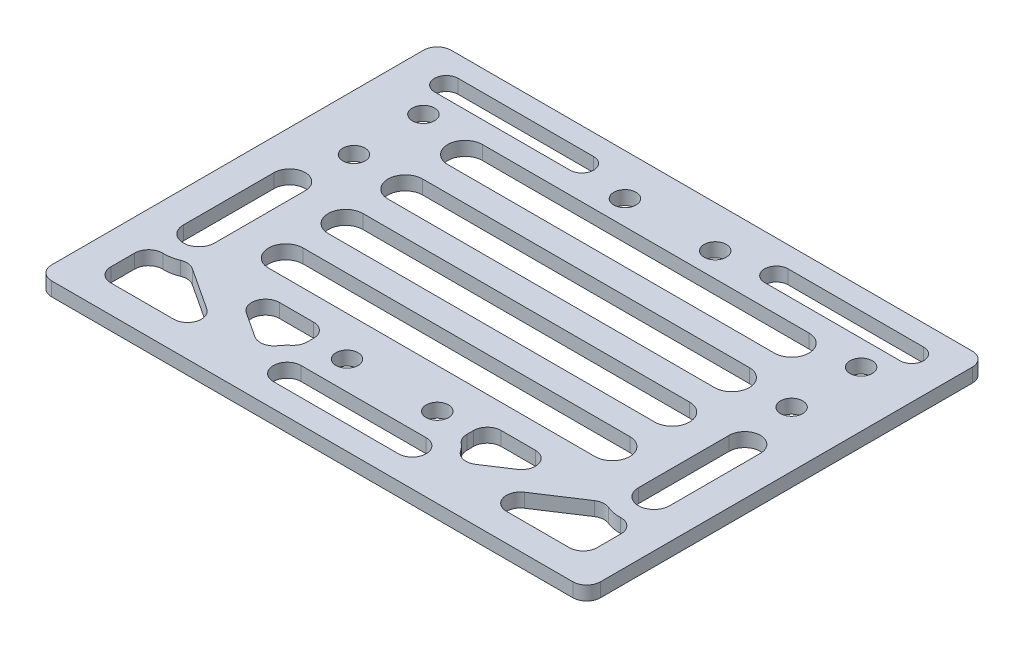
SolidWorks part; units mm, degrees
material "Thornel Mat VMA"
ref_plane "Front Plane" through (0, 0, 0) normal (0, 0, 1) x (1, 0, 0)
ref_plane "Top Plane" through (0, 0, 0) normal (0, 1, 0) x (1, 0, 0)
ref_plane "Right Plane" through (0, 0, 0) normal (1, 0, 0) x (0, 0, -1)
sketch "Sketch1" plane through (0, 0, 0) normal (0, 1, 0) x (1, 0, 0)
  line L0 (-31.5, 18.75) -> (-31.5, 8.75) construction
  line L1 (-39.5, 28.75) -> (39.5, 28.75)
  line L2 (-39.5, 28.75) -> (-39.5, -28.75)
  line L3 (-39.5, -28.75) -> (39.5, -28.75)
  line L4 (39.5, 28.75) -> (39.5, -28.75)
  line L5 (-39.5, 28.75) -> (39.5, -28.75) construction
  line L6 (-39.5, -28.75) -> (39.5, 28.75) construction
  line L7 (0, 28.75) -> (0, -28.75) construction
  line L8 (31.5, 18.75) -> (31.5, 8.75) construction
  line L9 (-6.5, 22.75) -> (6.5, 22.75) construction
  line L10 (-6.5, -17.25) -> (6.5, -17.25) construction
  circle A0 centre (-31.5, 18.75) radius 1.6
  circle A1 centre (-31.5, 8.75) radius 1.6
  circle A2 centre (31.5, 8.75) radius 1.6
  circle A3 centre (31.5, 18.75) radius 1.6
  circle A4 centre (-6.5, 22.75) radius 1.6
  circle A5 centre (-6.5, -17.25) radius 1.6
  circle A6 centre (6.5, 22.75) radius 1.6
  circle A7 centre (6.5, -17.25) radius 1.6
  point P0 (0, 0)
  dimension "D3" = 3.2
  dimension "D7" = 13
  dimension "D1" = 79
  dimension "D2" = 57.5
  dimension "D4" = 8
  dimension "D5" = 37.5
  dimension "D6" = 10
  dimension "D8" = 11.5
  dimension "D9" = 6
extrude "Boss-Extrude1" add sketch "Sketch1" along normal blind 2
sketch "Sketch2" plane through (0, 2, 0) normal (0, 1, 0) x (1, 0, 0)
  line L0 (0, 28.75) -> (0, -28.75) construction
  line L1 (39.5, 28.75) -> (-39.5, 28.75) construction
  line L2 (-39.5, -28.75) -> (39.5, -28.75) construction
  line L3 (-23.5, 16.75) -> (23.5, 16.75) construction
  line L4 (-23.5, 19.25) -> (23.5, 19.25)
  line L5 (-23.5, 14.25) -> (23.5, 14.25)
  line L6 (-6.5, 22.75) -> (6.5, 22.75) construction
  line L7 (-6.5, -17.25) -> (6.5, -17.25) construction
  line L8 (-31.5, 18.75) -> (-31.5, 8.75) construction
  line L9 (31.5, 18.75) -> (31.5, 8.75) construction
  line L10 (-23.5, 8.15) -> (23.5, 8.15) construction
  line L11 (-23.5, 10.65) -> (23.5, 10.65)
  line L12 (-23.5, 5.65) -> (23.5, 5.65)
  line L13 (-23.5, -0.45) -> (23.5, -0.45) construction
  line L14 (-23.5, 2.05) -> (23.5, 2.05)
  line L15 (-23.5, -2.95) -> (23.5, -2.95)
  line L16 (-23.5, -9.05) -> (23.5, -9.05) construction
  line L19 (-23.5, -6.55) -> (23.5, -6.55)
  line L24 (-39.5, 28.75) -> (-39.5, -28.75) construction
  line L25 (-33.5, 24.05) -> (-14, 24.05) construction
  line L26 (-33.5, 25.75) -> (-14, 25.75)
  line L27 (-33.5, 22.35) -> (-14, 22.35)
  line L28 (33.5, 24.05) -> (14, 24.05) construction
  line L29 (33.5, 25.75) -> (14, 25.75)
  line L30 (33.5, 22.35) -> (14, 22.35)
  line L31 (-23.5, -11.55) -> (23.5, -11.55)
  line L32 (-9, -23.35) -> (9, -23.35) construction
  line L33 (-9, -21.35) -> (9, -21.35)
  line L34 (-9, -25.35) -> (9, -25.35)
  line L35 (-32.75, 0.75) -> (-32.75, -12.3054) construction
  line L36 (-30.5, 0.75) -> (-30.5, -12.3054)
  line L37 (-35, 0.75) -> (-35, -12.3054)
  line L38 (32.75, 0.75) -> (32.75, -12.3054) construction
  line L39 (30.5, 0.75) -> (30.5, -12.3054)
  line L40 (35, 0.75) -> (35, -12.3054)
  line L41 (-35, -16.7705) -> (-35, -24.75)
  line L42 (-35, -24.75) -> (-17.2613, -24.75)
  line L43 (-25.1093, -15.05) -> (-11.5, -15.05)
  line L44 (-11.5, -15.05) -> (-11.5, -19.0199)
  line L45 (-28.5706, -15.05) -> (-13.8, -24.75) construction
  line L46 (-17.2613, -24.75) -> (-29.9271, -16.4323)
  line L47 (-13.9098, -22.4048) -> (-25.1093, -15.05)
  line L48 (17.2613, -24.75) -> (29.9271, -16.4323)
  line L49 (35, -24.75) -> (17.2613, -24.75)
  line L50 (35, -16.7705) -> (35, -24.75)
  line L51 (25.1093, -15.05) -> (11.5, -15.05)
  line L52 (13.9098, -22.4048) -> (25.1093, -15.05)
  line L53 (11.5, -15.05) -> (11.5, -19.0199)
  arc A0 (-23.5, 19.25) -> (-23.5, 14.25) centre (-23.5, 16.75) ccw
  arc A1 (23.5, 14.25) -> (23.5, 19.25) centre (23.5, 16.75) ccw
  arc A2 (-23.5, 10.65) -> (-23.5, 5.65) centre (-23.5, 8.15) ccw
  arc A3 (23.5, 5.65) -> (23.5, 10.65) centre (23.5, 8.15) ccw
  arc A4 (-23.5, 2.05) -> (-23.5, -2.95) centre (-23.5, -0.45) ccw
  arc A5 (23.5, -2.95) -> (23.5, 2.05) centre (23.5, -0.45) ccw
  arc A12 (-33.5, 25.75) -> (-33.5, 22.35) centre (-33.5, 24.05) ccw
  arc A13 (-14, 22.35) -> (-14, 25.75) centre (-14, 24.05) ccw
  arc A14 (33.5, 25.75) -> (33.5, 22.35) centre (33.5, 24.05) cw
  arc A15 (14, 22.35) -> (14, 25.75) centre (14, 24.05) cw
  arc A16 (-23.5, -6.55) -> (-23.5, -11.55) centre (-23.5, -9.05) ccw
  arc A17 (23.5, -11.55) -> (23.5, -6.55) centre (23.5, -9.05) ccw
  arc A18 (-9, -21.35) -> (-9, -25.35) centre (-9, -23.35) ccw
  arc A19 (9, -25.35) -> (9, -21.35) centre (9, -23.35) ccw
  arc A20 (-30.5, 0.75) -> (-35, 0.75) centre (-32.75, 0.75) ccw
  arc A21 (-35, -12.3054) -> (-30.5, -12.3054) centre (-32.75, -12.3054) ccw
  arc A22 (30.5, 0.75) -> (35, 0.75) centre (32.75, 0.75) cw
  arc A23 (35, -12.3054) -> (30.5, -12.3054) centre (32.75, -12.3054) cw
  arc A24 (-35, -16.7705) -> (-29.9271, -16.4323) centre (-32.75, -12.3054) ccw
  arc A25 (-11.5, -19.0199) -> (-13.9098, -22.4048) centre (-9, -23.35) ccw
  arc A26 (35, -16.7705) -> (29.9271, -16.4323) centre (32.75, -12.3054) cw
  arc A27 (11.5, -19.0199) -> (13.9098, -22.4048) centre (9, -23.35) cw
  point P8 (0, 16.75)
  point P32 (0, 8.15)
  point P39 (0, -0.45)
  point P45 (0, -9.05)
  point P52 (0, -23.35)
  point P61 (-23.75, 24.05)
  point P68 (23.75, 24.05)
  point P75 (-32.75, -5.7777)
  point P82 (32.75, -5.7777)
  dimension "D2" = 2.5
  dimension "D15" = 4
  dimension "D16" = 5
  dimension "D17" = 5
  dimension "D1" = 3.5
  dimension "D3" = 8
  dimension "D5" = 4
  dimension "D6" = 3.4
  dimension "D7" = 3.6
  dimension "D8" = 4.5
  dimension "D9" = 3
  dimension "D10" = 28
  dimension "D11" = 3.4
  dimension "D12" = 6
  dimension "D13" = 4.5
  dimension "D14" = 8
  dimension "D18" = 18
  dimension "D19" = 3.5
  dimension "D20" = 5
  dimension "D21" = 3.8
  dimension "D4" = 4
extrude "Cut-Extrude1" cut sketch "Sketch2" against normal through all
fillet "R2 Fillet 1" radius 2 20 edges at (39.5, 1, 28.75) (-39.5, 1, -28.75) (39.5, 1, -28.75) (-39.5, 1, 28.75) (35, 1, 24.75) (17.2613, 1, 24.75) (29.9271, 1, 16.4323) (35, 1, 16.7705) (11.5, 1, 19.0199) (11.5, 1, 15.05) (25.1093, 1, 15.05) (13.9098, 1, 22.4048) (-17.2613, 1, 24.75) (-35, 1, 24.75) (-29.9271, 1, 16.4323) (-13.9098, 1, 22.4048) (-25.1093, 1, 15.05) (-11.5, 1, 15.05) (-11.5, 1, 19.0199) (-35, 1, 16.7705)
